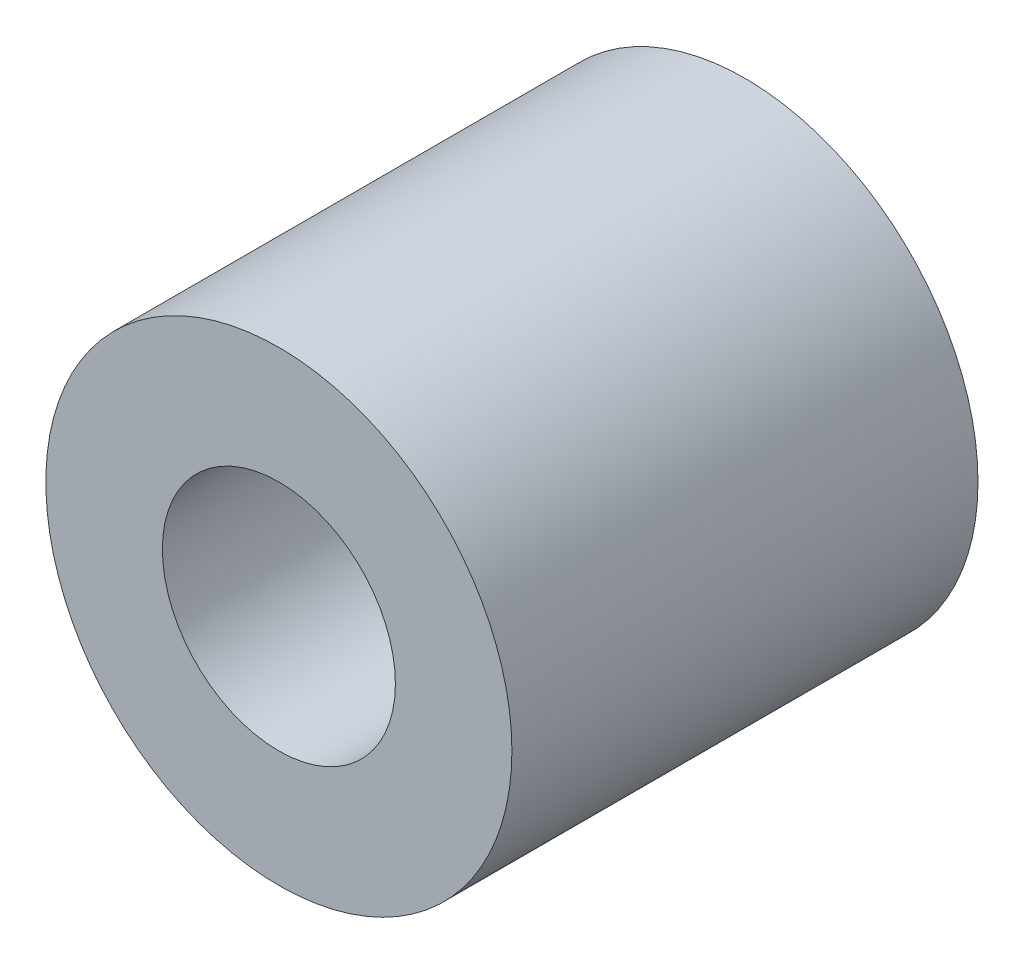
SolidWorks part; units mm, degrees
ref_plane "前视基准面" through (0, 0, 0) normal (0, 0, 1) x (1, 0, 0)
ref_plane "上视基准面" through (0, 0, 0) normal (0, 1, 0) x (1, 0, 0)
ref_plane "右视基准面" through (0, 0, 0) normal (1, 0, 0) x (0, 0, -1)
sketch "草图1" plane through (0, 0, 0) normal (0, 0, 1) x (1, 0, 0)
  circle A0 centre (0, 0) radius 30
  dimension "D1" = 60
extrude "凸台-拉伸1" add sketch "草图1" along normal blind 60
sketch "草图2" plane through (0, 0, 60) normal (0, 0, 1) x (1, 0, 0)
  circle A0 centre (0, 0) radius 7
  dimension "D1" = 14
extrude "切除-拉伸1" cut sketch "草图2" against normal through all
sketch "草图3" plane through (0, 0, 60) normal (0, 0, 1) x (1, 0, 0)
  circle A0 centre (0, 0) radius 15
  dimension "D1" = 30
extrude "切除-拉伸2" cut sketch "草图3" against normal blind 30
